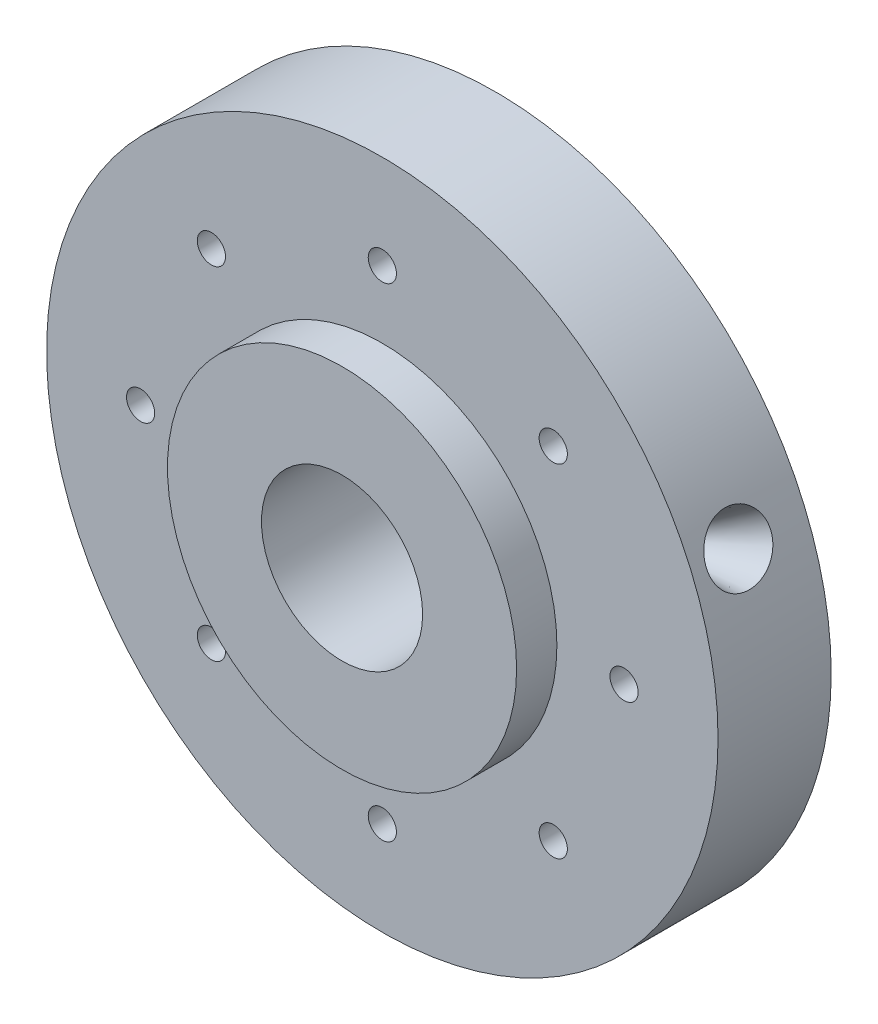
from build123d import *

# Parameters (mm, degrees)
SKETCH_1_R          = 125
SKETCH_1_R_2        = 5.25
EXTRUDE_1_DEPTH     = 42.13
SKETCH_2_R          = 65
EXTRUDE_2_DEPTH     = 15
SKETCH_3_R          = 30
CUT_EXTRUDE_1_DEPTH = 55
SKETCH_6_R          = 5
CUT_EXTRUDE_2_DEPTH = 50
SKETCH_7_R          = 9
CUT_EXTRUDE_3_DEPTH = 11


with BuildPart() as part:
    # 草图1 → 凸台-拉伸1 (new body)
    with BuildSketch(Plane.XY):
        Circle(SKETCH_1_R)
        with Locations((0, 90)):
            Circle(SKETCH_1_R_2, mode=Mode.SUBTRACT)
        with Locations((63.639610307, 63.639610307)):
            Circle(SKETCH_1_R_2, mode=Mode.SUBTRACT)
        with Locations((90, 0)):
            Circle(SKETCH_1_R_2, mode=Mode.SUBTRACT)
        with Locations((63.639610307, -63.639610307)):
            Circle(SKETCH_1_R_2, mode=Mode.SUBTRACT)
        with Locations((0, -90)):
            Circle(SKETCH_1_R_2, mode=Mode.SUBTRACT)
        with Locations((-63.639610307, -63.639610307)):
            Circle(SKETCH_1_R_2, mode=Mode.SUBTRACT)
        with Locations((-90, 0)):
            Circle(SKETCH_1_R_2, mode=Mode.SUBTRACT)
        with Locations((-63.639610307, 63.639610307)):
            Circle(SKETCH_1_R_2, mode=Mode.SUBTRACT)
    extrude(amount=EXTRUDE_1_DEPTH)

    # 草图2 → 凸台-拉伸2 (add)
    with BuildSketch(Plane.XY.offset(42.13)):
        Circle(SKETCH_2_R)
    extrude(amount=EXTRUDE_2_DEPTH)

    # 草图3 → 切除-拉伸1 (cut)
    with BuildSketch(Plane.XY.offset(57.13)):
        Circle(SKETCH_3_R)
    extrude(amount=-CUT_EXTRUDE_1_DEPTH, mode=Mode.SUBTRACT)

    # 草图5 → 切除-旋转1 (revolve, cut)
    with BuildSketch(Plane(origin=(0, 0, 0), x_dir=(0, 0, 1), z_dir=(-0.3826834323650906, 0.9238795325112865, 0)), mode=Mode.PRIVATE) as cut_revolve_1_sk:
        Polygon((30, 100.5), (37.70842723, 127.382480462), (25, 127.382480462), (25, 124.917518293), (25, 0), (30, 0), align=None)
    revolve(cut_revolve_1_sk.sketch.rotate(Axis((123.47749494, 51.146053052, 25), (-0.9238795325112864, -0.3826834323650906, 0)), 90), axis=Axis((123.47749494, 51.146053052, 25), (-0.9238795325112864, -0.3826834323650906, 0)), mode=Mode.SUBTRACT)

    # 草图6 → 切除-拉伸2 (cut)
    with BuildSketch(Plane.XY.offset(42.13)):
        with Locations((43.884277794, 18.177463037)):
            Circle(SKETCH_6_R)
    extrude(amount=-CUT_EXTRUDE_2_DEPTH, mode=Mode.SUBTRACT)

    # 草图7 → 切除-拉伸3 (cut)
    with BuildSketch(Plane(origin=(0, 0, 0), x_dir=(-1, 0, 0), z_dir=(0, 0, -1))):
        with Locations((0, 90)):
            Circle(SKETCH_7_R)
        with Locations((63.639610307, 63.639610307)):
            Circle(SKETCH_7_R)
        with Locations((90, 0)):
            Circle(SKETCH_7_R)
        with Locations((63.639610307, -63.639610307)):
            Circle(SKETCH_7_R)
        with Locations((0, -90)):
            Circle(SKETCH_7_R)
        with Locations((-63.639610307, -63.639610307)):
            Circle(SKETCH_7_R)
        with Locations((-90, 0)):
            Circle(SKETCH_7_R)
        with Locations((-63.639610307, 63.639610307)):
            Circle(SKETCH_7_R)
    extrude(amount=-CUT_EXTRUDE_3_DEPTH, mode=Mode.SUBTRACT)


solid = part.part
